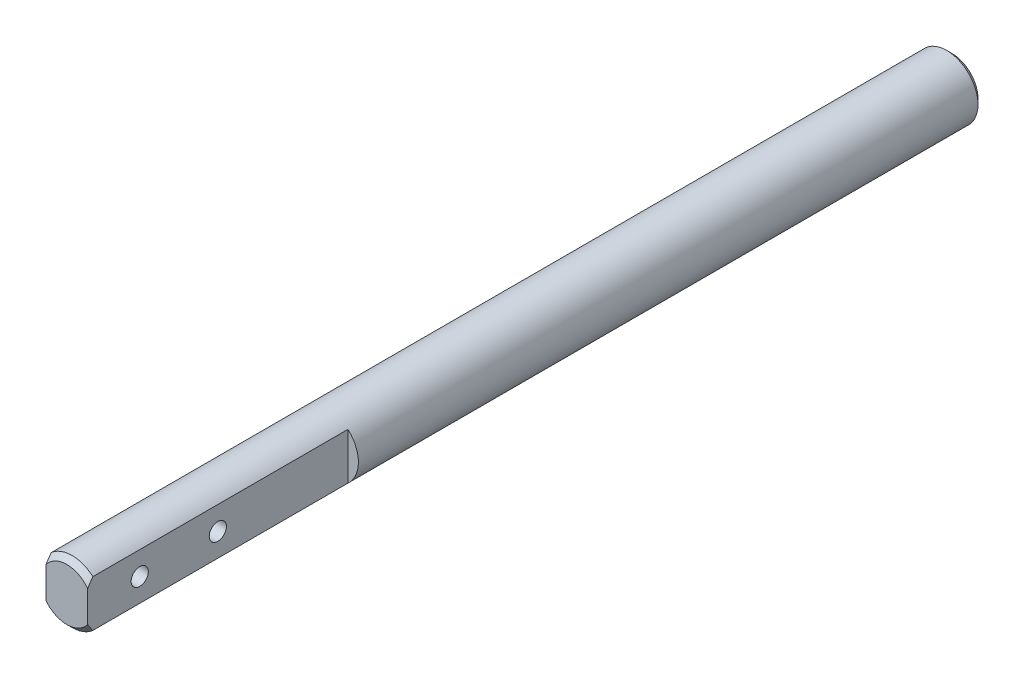
from build123d import *

# Parameters (mm, degrees)
SKETCH1_R                   = 6
BOSS_EXTRUDE1_DEPTH         = 170
CHAMFER1_SIZE               = 1
CUT_EXTRUDE1_DEPTH          = 171.211632975
CUT_EXTRUDE1_DEPTH_BACK     = 171.211632975
SKETCH2_W                   = 2
SKETCH2_H                   = 50
M4_TAPPED_HOLE1_D           = 3.3
M4_TAPPED_HOLE1_CSINK_D     = 4.05
M4_TAPPED_HOLE1_CSINK_ANGLE = 90


with BuildPart() as part:
    # Sketch1 → Boss-Extrude1 (new body)
    with BuildSketch(Plane.XY):
        Circle(SKETCH1_R)
    extrude(amount=BOSS_EXTRUDE1_DEPTH)

    # Chamfer1
    chamfer1_edges = [part.edges().sort_by_distance(p)[0] for p in [
        (-6, 0, 0),
        (-6, 0, 170),
    ]]
    chamfer(chamfer1_edges, length=CHAMFER1_SIZE)

    # Sketch2 → Cut-Extrude1 (cut, two sides: drawn at the far end of the back side and taken through both)
    with BuildSketch(Plane(origin=(0, 0, 0), x_dir=(1, 0, 0), z_dir=(0, 1, 0)).offset(-CUT_EXTRUDE1_DEPTH_BACK)):
        with Locations((-5, -145)):
            Rectangle(SKETCH2_W, SKETCH2_H)
        with Locations((5, -145)):
            Rectangle(SKETCH2_W, SKETCH2_H)
    extrude(amount=CUT_EXTRUDE1_DEPTH + CUT_EXTRUDE1_DEPTH_BACK, mode=Mode.SUBTRACT)

    # M4 Tapped Hole1 (through all)
    with Locations(Plane.ZY.offset(4)):
        with Locations((160, 0), (145, 0)):
            CounterSinkHole(M4_TAPPED_HOLE1_D / 2, M4_TAPPED_HOLE1_CSINK_D / 2, counter_sink_angle=M4_TAPPED_HOLE1_CSINK_ANGLE)


solid = part.part
